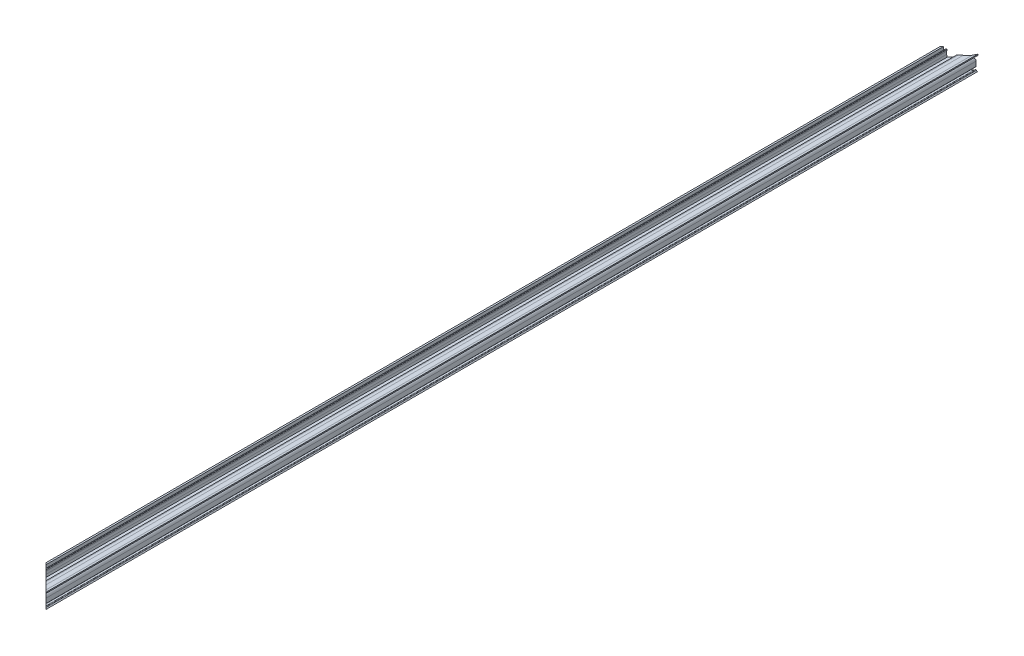
SolidWorks part; units mm, degrees
ref_plane "Front Plane" through (0, 0, 0) normal (0, 0, 1) x (1, 0, 0)
ref_plane "Top Plane" through (0, 0, 0) normal (0, 1, 0) x (1, 0, 0)
ref_plane "Right Plane" through (0, 0, 0) normal (1, 0, 0) x (0, 0, -1)
sketch "Sketch2" plane through (0, 0, 0) normal (0, 0, 1) x (1, 0, 0)
  line L0 (27.4296, 61.2035) -> (27.4296, 62.4835)
  line L1 (27.6297, 70.5806) -> (28.2239, 70.4974)
  line L2 (28.2521, 68.5355) -> (28.4794, 70.1587)
  line L3 (24.4296, 48.2035) -> (46.4296, 48.2035)
  line L4 (46.4296, 65.5674) -> (46.4296, 64.3068)
  line L5 (35.3196, 63.5648) -> (35.3196, 62.5671)
  line L6 (27.0637, 68.7019) -> (27.291, 70.3251)
  line L7 (28.6296, 62.5671) -> (34.1196, 62.5671)
  line L8 (24.4296, 73.2035) -> (26.4296, 73.2035)
  line L9 (43.408, 63.3348) -> (46.4296, 64.3068)
  line L10 (34.1196, 62.5671) -> (34.1196, 64.7671)
  line L11 (43.0405, 64.4771) -> (46.4296, 65.5674)
  line L13 (28.2521, 65.2634) -> (28.6296, 62.5671)
  line L14 (45.3996, 58.5671) -> (45.3996, 53.2529)
  line L15 (35.3196, 62.5671) -> (41.3996, 62.5671)
  line L16 (27.0637, 65.097) -> (27.4296, 62.4835)
  line L17 (34.1196, 64.7671) -> (35.1196, 64.7671)
  line L18 (24.4296, 48.2035) -> (24.4296, 73.2035)
  line L19 (26.4296, 73.2035) -> (26.4296, 61.2035)
  line L20 (26.4296, 61.2035) -> (27.4296, 61.2035)
  arc A0 (35.1196, 64.7671) -> (37.8501, 64.3871) centre (35.1196, 54.7671) cw
  arc A1 (28.4794, 70.1587) -> (28.2239, 70.4974) centre (28.1823, 70.2003) ccw
  arc A2 (37.8501, 64.3871) -> (43.0405, 64.4771) centre (40.2966, 73.0066) ccw
  arc A3 (27.0637, 65.097) -> (27.0637, 68.7019) centre (39.9382, 66.8995) cw
  arc A4 (27.291, 70.3251) -> (27.6297, 70.5806) centre (27.5881, 70.2835) cw
  arc A5 (37.5225, 63.2327) -> (43.408, 63.3348) centre (40.2966, 73.0066) ccw
  arc A6 (45.3996, 53.2529) -> (44.608, 52.8468) centre (44.8996, 53.2529) cw
  arc A7 (28.2521, 65.2634) -> (28.2521, 68.5355) centre (39.9382, 66.8995) cw
  arc A8 (44.608, 52.8468) -> (44.6629, 49.8013) centre (43.4996, 51.3035) ccw
  arc A9 (45.3996, 58.5671) -> (41.3996, 62.5671) centre (41.3996, 58.5671) ccw
  arc A10 (45.4401, 49.3477) -> (44.6629, 49.8013) centre (44.96, 49.4177) ccw
  arc A11 (35.3196, 63.5648) -> (37.5225, 63.2327) centre (35.1196, 54.7671) cw
  arc A12 (45.4401, 49.3477) -> (46.4296, 48.2035) centre (46.4296, 49.2035) ccw
  dimension "D7" = 4
  dimension "D9" = 3.8
  dimension "D10" = 2
  dimension "D4" = 0.3
  dimension "D5" = 0.3
  dimension "D12" = 0.5
  dimension "D3" = 1
  dimension "D11" = 3.1
extrude "Extrude1" add sketch "Sketch2" along normal blind 1081
sketch "Sketch4" plane through (0, 48.2035, 0) normal (0, -1, 0) x (1, 0, 0)
  line L4 (46.4296, 0) -> (24.4296, 22)
  line L5 (24.4296, 22) -> (24.4296, 0)
  line L6 (24.4296, 1081) -> (24.4296, 0) construction
  line L7 (24.4296, 1081) -> (24.5231, 1081.0914)
  dimension "D1" = 45
extrude "Extrude4" cut sketch "Sketch4" against normal through all and the other way through all contours L4 L5
sketch "Sketch5" plane through (0, 48.2035, 0) normal (0, -1, 0) x (1, 0, 0)
  line L0 (46.4296, 1081) -> (24.4296, 1059)
  line L1 (24.4296, 1081) -> (24.4296, 22) construction
  line L2 (24.4296, 1059) -> (24.4296, 1081)
  line L3 (24.4296, 1081) -> (46.4296, 1081)
  dimension "D1" = 45
extrude "Extrude5" cut sketch "Sketch5" against normal blind 30
